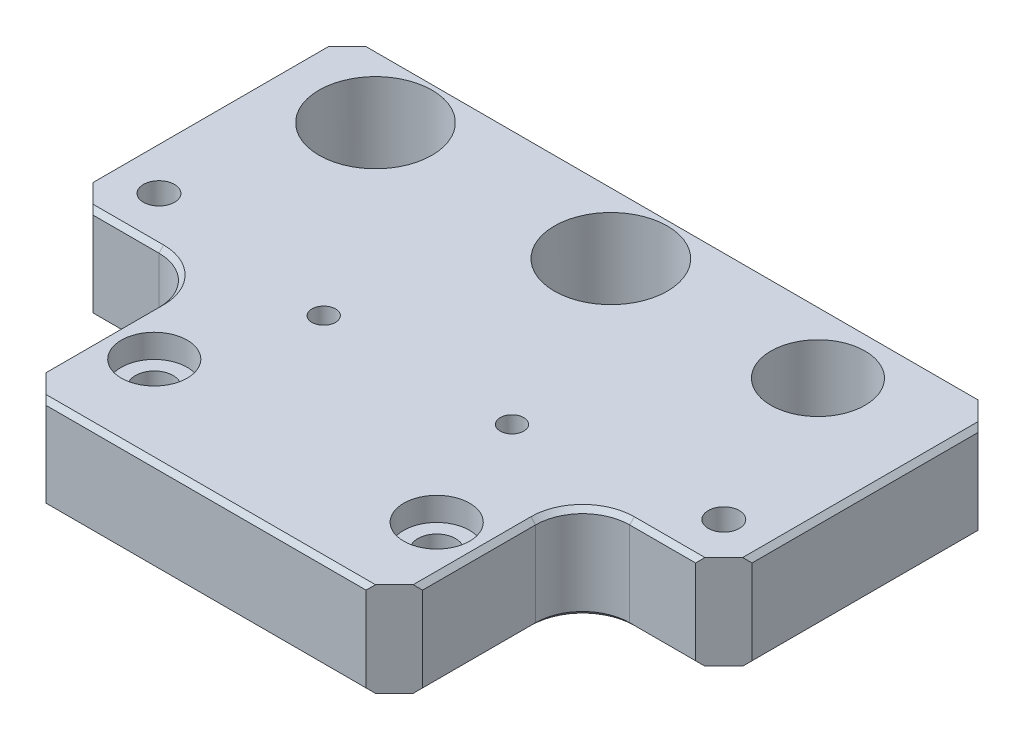
from build123d import *

# Parameters (mm, degrees)
SKETCH1_W           = 70
SKETCH1_H           = 30
BOSS_EXTRUDE1_DEPTH = 10
SKETCH8_R           = 5
CUT_EXTRUDE6_DEPTH  = 11
SKETCH9_R           = 6
CUT_EXTRUDE7_DEPTH  = 11
M4_TAPPED_HOLE2_D   = 3.3
SKETCH13_W          = 40
SKETCH13_H          = 10
BOSS_EXTRUDE2_DEPTH = 20
SKETCH14_R          = 2
CUT_EXTRUDE8_DEPTH  = 77.811457479
M3_TAPPED_HOLE1_D   = 2.5
CHAMFER3_SIZE       = 3
FILLET1_R           = 5
CHAMFER4_SIZE       = 0.5
SKETCH18_R          = 3.5
CUT_EXTRUDE9_DEPTH  = 2.5
CUT_EXTRUDE10_START = -2.5
SKETCH19_R          = 3.5
CUT_EXTRUDE10_DEPTH = 2.5


with BuildPart() as part:
    # Sketch1 → Boss-Extrude1 (new body)
    with BuildSketch(Plane(origin=(0, 0, 0), x_dir=(1, 0, 0), z_dir=(0, 1, 0))):
        with Locations((-35, 15)):
            Rectangle(SKETCH1_W, SKETCH1_H)
    extrude(amount=BOSS_EXTRUDE1_DEPTH)

    # Sketch8 → Cut-Extrude6 (cut)
    with BuildSketch(Plane.XZ):
        with Locations(Location((-13, -23, 0), (0, 0, 270))):
            Circle(SKETCH8_R)
    extrude(amount=-CUT_EXTRUDE6_DEPTH, mode=Mode.SUBTRACT)

    # Sketch9 → Cut-Extrude7 (cut)
    with BuildSketch(Plane.XZ):
        with Locations(Location((-60, -23, 0), (0, 0, 270))):
            Circle(SKETCH9_R)
        with Locations(Location((-35, -23, 0), (0, 0, 270))):
            Circle(SKETCH9_R)
    extrude(amount=-CUT_EXTRUDE7_DEPTH, mode=Mode.SUBTRACT)

    # M4 Tapped Hole2 (through all)
    with Locations(Plane(origin=(0, 0, 0), x_dir=(-1, 0, 0), z_dir=(0, -1, 0))):
        with Locations((65, 5), (5, 5)):
            Hole(M4_TAPPED_HOLE2_D / 2)

    # Sketch13 → Boss-Extrude2 (add)
    with BuildSketch(Plane.XY):
        with Locations((-35, 5)):
            Rectangle(SKETCH13_W, SKETCH13_H)
    extrude(amount=BOSS_EXTRUDE2_DEPTH)

    # Sketch14 → Cut-Extrude8 (cut, through all)
    with BuildSketch(Plane(origin=(0, 10, 0), x_dir=(1, 0, 0), z_dir=(0, 1, 0))):
        with Locations(Location((-50, -10.5, 0), (0, 0, 270))):
            Circle(SKETCH14_R)
        with Locations(Location((-20, -10.5, 0), (0, 0, 270))):
            Circle(SKETCH14_R)
    extrude(amount=-CUT_EXTRUDE8_DEPTH, mode=Mode.SUBTRACT)

    # M3 Tapped Hole1 (through all)
    with Locations(Plane(origin=(0, 0, 0), x_dir=(-1, 0, 0), z_dir=(0, -1, 0))):
        with Locations((25, 2.5), (45, 2.5)):
            Hole(M3_TAPPED_HOLE1_D / 2)

    # Chamfer3
    chamfer3_edges = [part.edges().sort_by_distance(p)[0] for p in [
        (0, 5, -30),
        (0, 5, 0),
        (-15, 5, 20),
        (-55, 5, 20),
        (-70, 5, 0),
        (-70, 5, -30),
    ]]
    chamfer(chamfer3_edges, length=CHAMFER3_SIZE)

    # Fillet1
    fillet1_edges = [part.edges().sort_by_distance(p)[0] for p in [
        (-15, 5, 0),
        (-55, 5, 0),
    ]]
    fillet(fillet1_edges, radius=FILLET1_R)

    # Chamfer4
    chamfer4_edges = [part.edges().sort_by_distance(p)[0] for p in [
        (-6.5, 0, 0),
        (-6.5, 10, 0),
        (-13.535533906, 10, 1.464466094),
        (-13.535533906, 0, 1.464466094),
        (-56.464466094, 0, 1.464466094),
        (-56.464466094, 10, 1.464466094),
        (-35, 0, -30),
        (-35, 10, -30),
        (-70, 0, -15),
        (0, 0, -15),
        (-15, 0, 11),
        (-35, 0, 20),
        (-55, 0, 11),
        (-63.5, 0, 0),
        (0, 10, -15),
        (-70, 10, -15),
        (-63.5, 10, 0),
        (-55, 10, 11),
        (-35, 10, 20),
        (-15, 10, 11),
    ]]
    chamfer(chamfer4_edges, length=CHAMFER4_SIZE)

    # Sketch18 → Cut-Extrude9 (cut)
    with BuildSketch(Plane(origin=(0, 10, 0), x_dir=(1, 0, 0), z_dir=(0, 1, 0))):
        with Locations(Location((-50, -10.5, 0), (0, 0, 270))):
            Circle(SKETCH18_R)
        with Locations(Location((-20, -10.5, 0), (0, 0, 270))):
            Circle(SKETCH18_R)
    extrude(amount=-CUT_EXTRUDE9_DEPTH, mode=Mode.SUBTRACT)

    # Sketch19 → Cut-Extrude10 (cut)
    with BuildSketch(Plane.XZ.offset(CUT_EXTRUDE10_START)):
        with Locations(Location((-50, 10.5, 0), (0, 0, 90))):
            Circle(SKETCH19_R)
        with Locations(Location((-20, 10.5, 0), (0, 0, 90))):
            Circle(SKETCH19_R)
    extrude(amount=CUT_EXTRUDE10_DEPTH, mode=Mode.SUBTRACT)


solid = part.part
